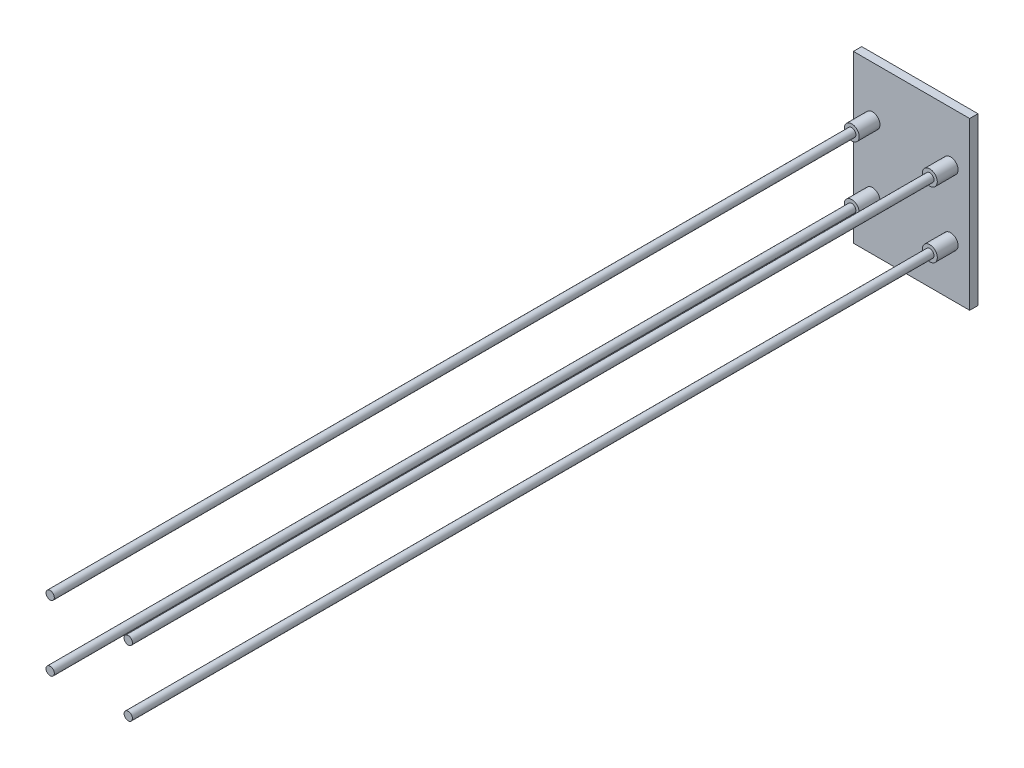
from build123d import *

# Parameters (mm, degrees)
SKETCH2_W           = 140
SKETCH2_H           = 200
SKETCH2_R           = 5
BOSS_EXTRUDE1_DEPTH = 10
SKETCH3_R           = 9
SKETCH3_R_2         = 5
BOSS_EXTRUDE2_DEPTH = 25
SKETCH4_R           = 5
BOSS_EXTRUDE3_DEPTH = 1000


with BuildPart() as part:
    # Sketch2 → Boss-Extrude1 (new body)
    with BuildSketch(Plane.XY):
        Rectangle(SKETCH2_W, SKETCH2_H)
        with Locations((-47, 39.5)):
            Circle(SKETCH2_R, mode=Mode.SUBTRACT)
        with Locations((-47, -39.5)):
            Circle(SKETCH2_R, mode=Mode.SUBTRACT)
        with Locations((47, 39.5)):
            Circle(SKETCH2_R, mode=Mode.SUBTRACT)
        with Locations((47, -39.5)):
            Circle(SKETCH2_R, mode=Mode.SUBTRACT)
    extrude(amount=BOSS_EXTRUDE1_DEPTH)

    # Sketch3 → Boss-Extrude2 (add)
    # profile 1 of 4: a face of its own
    with BuildSketch(Plane.XY.offset(10)):
        with Locations((-47, 39.5)):
            Circle(SKETCH3_R)
        with Locations((-47, 39.5)):
            Circle(SKETCH3_R_2, mode=Mode.SUBTRACT)
    # profile 2 of 4: a face of its own
    with BuildSketch(Plane.XY.offset(10)):
        with Locations((47, 39.5)):
            Circle(SKETCH3_R)
        with Locations((47, 39.5)):
            Circle(SKETCH3_R_2, mode=Mode.SUBTRACT)
    # profile 3 of 4: a face of its own
    with BuildSketch(Plane.XY.offset(10)):
        with Locations((47, -39.5)):
            Circle(SKETCH3_R)
        with Locations((47, -39.5)):
            Circle(SKETCH3_R_2, mode=Mode.SUBTRACT)
    # profile 4 of 4: a face of its own
    with BuildSketch(Plane.XY.offset(10)):
        with Locations((-47, -39.5)):
            Circle(SKETCH3_R)
        with Locations((-47, -39.5)):
            Circle(SKETCH3_R_2, mode=Mode.SUBTRACT)
    extrude(amount=BOSS_EXTRUDE2_DEPTH)

    # Sketch4 → Boss-Extrude3 (add)
    with BuildSketch(Plane(origin=(0, 0, 0), x_dir=(-1, 0, 0), z_dir=(0, 0, -1))):
        with Locations((-47, 39.5)):
            Circle(SKETCH4_R)
        with Locations((47, 39.5)):
            Circle(SKETCH4_R)
        with Locations((47, -39.5)):
            Circle(SKETCH4_R)
        with Locations((-47, -39.5)):
            Circle(SKETCH4_R)
    extrude(amount=-BOSS_EXTRUDE3_DEPTH)


solid = part.part
